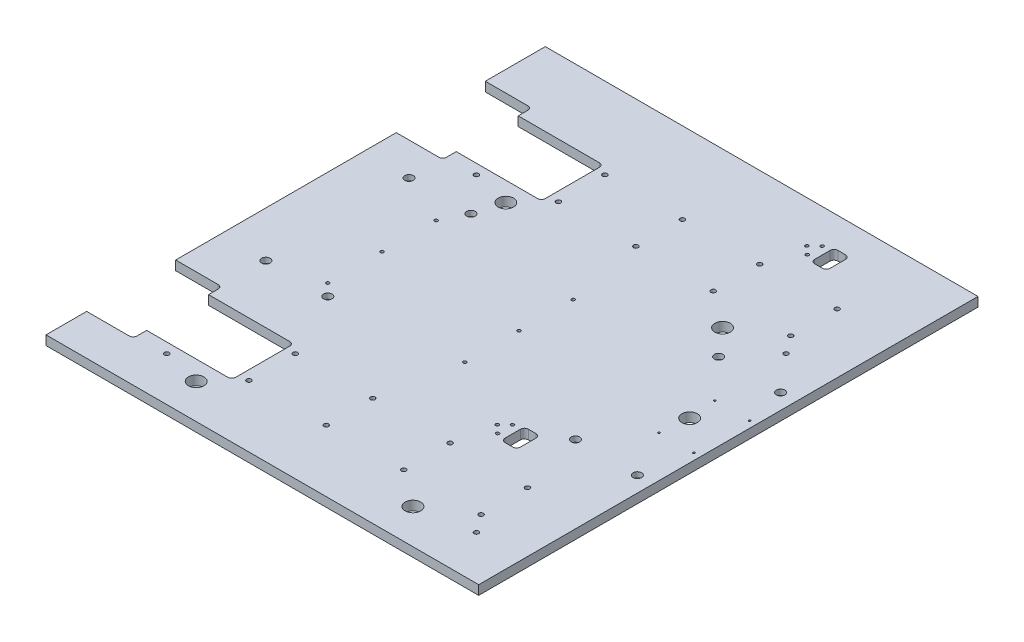
from build123d import *

# Parameters (mm, degrees)
SKETCH1_W                                         = 559
SKETCH1_H                                         = 645
EXTRUDE1_DEPTH                                    = 6
SKETCH2_W                                         = 170
SKETCH2_H                                         = 80
CUT_EXTRUDE1_DEPTH                                = 427.931493334
SKETCH3_W                                         = 60
SKETCH3_H                                         = 115
CUT_EXTRUDE2_DEPTH                                = 427.931493334
FILLET1_R                                         = 5
M6_SOCKET_HEAD_CAP_SCREW_COUNTERBORE1_D           = 6.6
M6_SOCKET_HEAD_CAP_SCREW_COUNTERBORE1_CBORE_D     = 11
M6_SOCKET_HEAD_CAP_SCREW_COUNTERBORE1_CBORE_DEPTH = 7
M3_TAPPED_HOLE1_D                                 = 2.5
M3_TAPPED_HOLE1_DEPTH                             = 9.5
M3_TAPPED_HOLE1_TIP                               = 0.751075774
M5_TAPPED_HOLE1_D                                 = 4.2
M5_TAPPED_HOLE2_D                                 = 4.2
SKETCH12_W                                        = 20
SKETCH12_H                                        = 30
CUT_EXTRUDE3_DEPTH                                = 427.931493334
FILLET2_R                                         = 5
SKETCH13_R                                        = 10
CUT_EXTRUDE4_DEPTH                                = 427.931493334
SKETCH14_R                                        = 10
CUT_EXTRUDE5_DEPTH                                = 427.931493334
LINEAR_PATTERN1_COUNT                             = 2
LINEAR_PATTERN1_PITCH                             = 400
SKETCH15_R                                        = 3
CUT_EXTRUDE6_DEPTH                                = 427.931493334
SKETCH17_R                                        = 3
CUT_EXTRUDE7_DEPTH                                = 427.931493334


with BuildPart() as part:
    # Sketch1 → Extrude1 (new, symmetric)
    with BuildSketch(Plane(origin=(0, 0, 0), x_dir=(1, 0, 0), z_dir=(0, 1, 0))):
        Rectangle(SKETCH1_W, SKETCH1_H)
    extrude(amount=EXTRUDE1_DEPTH, both=True)

    # Sketch2 → Cut-Extrude1 (cut, through all)
    with BuildSketch(Plane(origin=(0, 6, 0), x_dir=(1, 0, 0), z_dir=(0, 1, 0))):
        with Locations((-194.5, -212.5)):
            Rectangle(SKETCH2_W, SKETCH2_H)
        with Locations((-194.5, 187.5)):
            Rectangle(SKETCH2_W, SKETCH2_H)
    extrude(amount=-CUT_EXTRUDE1_DEPTH, mode=Mode.SUBTRACT)

    # Sketch3 → Cut-Extrude2 (cut, through all)
    with BuildSketch(Plane(origin=(0, 6, 0), x_dir=(1, 0, 0), z_dir=(0, 1, 0))):
        with Locations((-249.5, 187.5)):
            Rectangle(SKETCH3_W, SKETCH3_H)
        with Locations((-249.5, -212.5)):
            Rectangle(SKETCH3_W, SKETCH3_H)
    extrude(amount=-CUT_EXTRUDE2_DEPTH, mode=Mode.SUBTRACT)

    # Fillet1
    fillet1_edges = [part.edges().sort_by_distance(p)[0] for p in [
        (-109.5, 0, 172.5),
        (-109.5, 0, 252.5),
        (-109.5, 0, -147.5),
        (-109.5, 0, -227.5),
        (-219.5, 0, -245),
        (-219.5, 0, -130),
        (-219.5, 0, 155),
        (-219.5, 0, 270),
    ]]
    fillet(fillet1_edges, radius=FILLET1_R)

    # M6 Socket Head Cap Screw Counterbore1 (through all)
    with Locations(Plane(origin=(-220.5, 6, -87.5), x_dir=(0, 0, 1), z_dir=(0, 1, 0))):
        with Locations((0, 0), (185, 0), (185, 80), (0, 80), (185, 400), (185, 480), (0, 400), (0, 480)):
            CounterBoreHole(M6_SOCKET_HEAD_CAP_SCREW_COUNTERBORE1_D / 2, M6_SOCKET_HEAD_CAP_SCREW_COUNTERBORE1_CBORE_D / 2, M6_SOCKET_HEAD_CAP_SCREW_COUNTERBORE1_CBORE_DEPTH)

    # M3 Tapped Hole1
    with Locations(Plane(origin=(271, 6, -36), x_dir=(0, 0, 1), z_dir=(0, 1, 0))):
        with Locations((0, 0), (0, -45), (72, 0), (72, -45)):
            Hole(M3_TAPPED_HOLE1_D / 2, depth=M3_TAPPED_HOLE1_DEPTH)
            with Locations((0, 0, -(M3_TAPPED_HOLE1_DEPTH + M3_TAPPED_HOLE1_TIP / 2))):  # 118° drill point
                Cone(0, M3_TAPPED_HOLE1_D / 2, M3_TAPPED_HOLE1_TIP, mode=Mode.SUBTRACT)

    # M5 Tapped Hole1 (through all)
    with Locations(Plane(origin=(122.5, 6, 141.1), x_dir=(0, 0, 1), z_dir=(0, 1, 0))):
        with Locations((0, 0), (-9.6, -10), (-19.2, 0), (-409.6, -10), (-400, 0), (-419.2, 0)):
            Hole(M5_TAPPED_HOLE1_D / 2)

    # M5 Tapped Hole2 (through all)
    with Locations(Plane(origin=(-155.5, 6, 82.5), x_dir=(0, 0, 1), z_dir=(0, 1, 0))):
        with Locations((0, 0), (-140, 0), (0, 177), (-140, 177), (-70, 0), (-70, 177)):
            Hole(M5_TAPPED_HOLE2_D / 2)

    # Sketch12 → Cut-Extrude3 (cut, through all)
    with BuildSketch(Plane(origin=(0, 6, 0), x_dir=(1, 0, 0), z_dir=(0, 1, 0))):
        with Locations((142.5, -131.5)):
            Rectangle(SKETCH12_W, SKETCH12_H)
        with Locations((142.5, 268.5)):
            Rectangle(SKETCH12_W, SKETCH12_H)
    extrude(amount=-CUT_EXTRUDE3_DEPTH, mode=Mode.SUBTRACT)

    # Fillet2
    fillet2_edges = [part.edges().sort_by_distance(p)[0] for p in [
        (132.5, 0, -253.5),
        (132.5, 0, -283.5),
        (152.5, 0, -283.5),
        (152.5, 0, -253.5),
        (132.5, 0, 116.5),
        (152.5, 0, 116.5),
        (152.5, 0, 146.5),
        (132.5, 0, 146.5),
    ]]
    fillet(fillet2_edges, radius=FILLET2_R)

    # Sketch13 → Cut-Extrude4 (cut, through all)
    with BuildSketch(Plane(origin=(0, 6, 0), x_dir=(1, 0, 0), z_dir=(0, 1, 0))):
        with Locations(Location((229.5, 0, 0), (0, 0, 270))):
            Circle(SKETCH13_R)
    extrude(amount=-CUT_EXTRUDE4_DEPTH, mode=Mode.SUBTRACT)

    # Sketch14 → Cut-Extrude5 (cut, through all)
    with BuildSketch(Plane(origin=(0, 6, 0), x_dir=(1, 0, 0), z_dir=(0, 1, 0))):
        with Locations(Location((-130.5, 122.5, 0), (0, 0, 270))):
            Circle(SKETCH14_R)
        with Locations(Location((149.5, 122.5, 0), (0, 0, 270))):
            Circle(SKETCH14_R)
    cut_extrude5 = extrude(amount=-CUT_EXTRUDE5_DEPTH, mode=Mode.SUBTRACT)

    # Linear Pattern1: Cut-Extrude5 ×2
    with Locations(*[(0, 0, i * LINEAR_PATTERN1_PITCH) for i in range(1, LINEAR_PATTERN1_COUNT)]):
        add(cut_extrude5, mode=Mode.SUBTRACT)

    # Sketch15 → Cut-Extrude6 (cut, through all)
    with BuildSketch(Plane(origin=(0, 6, 0), x_dir=(1, 0, 0), z_dir=(0, 1, 0))):
        with Locations(Location((-180.5, 134.5, 0), (0, 0, 270))):
            Circle(SKETCH15_R)
        with Locations(Location((219.5, 134.5, 0), (0, 0, 270))):
            Circle(SKETCH15_R)
        with Locations(Location((219.5, -265.5, 0), (0, 0, 270))):
            Circle(SKETCH15_R)
        with Locations(Location((-180.5, -265.5, 0), (0, 0, 270))):
            Circle(SKETCH15_R)
    extrude(amount=-CUT_EXTRUDE6_DEPTH, mode=Mode.SUBTRACT)

    # Sketch17 → Cut-Extrude7 (cut, through all)
    with BuildSketch(Plane.XZ.offset(6)):
        with Locations(Location((202.5, 242.5, 0), (0, 0, 270))):
            Circle(SKETCH17_R)
        with Locations(Location((202.5, 182.5, 0), (0, 0, 270))):
            Circle(SKETCH17_R)
        with Locations(Location((102.5, 242.5, 0), (0, 0, 270))):
            Circle(SKETCH17_R)
        with Locations(Location((102.5, 182.5, 0), (0, 0, 270))):
            Circle(SKETCH17_R)
        with Locations(Location((2.5, 242.5, 0), (0, 0, 270))):
            Circle(SKETCH17_R)
        with Locations(Location((2.5, 182.5, 0), (0, 0, 270))):
            Circle(SKETCH17_R)
        with Locations(Location((-97.5, 242.5, 0), (0, 0, 270))):
            Circle(SKETCH17_R)
        with Locations(Location((-97.5, 182.5, 0), (0, 0, 270))):
            Circle(SKETCH17_R)
        with Locations(Location((-97.5, -157.5, 0), (0, 0, 270))):
            Circle(SKETCH17_R)
        with Locations(Location((-97.5, -217.5, 0), (0, 0, 270))):
            Circle(SKETCH17_R)
        with Locations(Location((2.5, -157.5, 0), (0, 0, 270))):
            Circle(SKETCH17_R)
        with Locations(Location((2.5, -217.5, 0), (0, 0, 270))):
            Circle(SKETCH17_R)
        with Locations(Location((102.5, -157.5, 0), (0, 0, 270))):
            Circle(SKETCH17_R)
        with Locations(Location((102.5, -217.5, 0), (0, 0, 270))):
            Circle(SKETCH17_R)
        with Locations(Location((202.5, -157.5, 0), (0, 0, 270))):
            Circle(SKETCH17_R)
        with Locations(Location((202.5, -217.5, 0), (0, 0, 270))):
            Circle(SKETCH17_R)
    extrude(amount=-CUT_EXTRUDE7_DEPTH, mode=Mode.SUBTRACT)


solid = part.part
